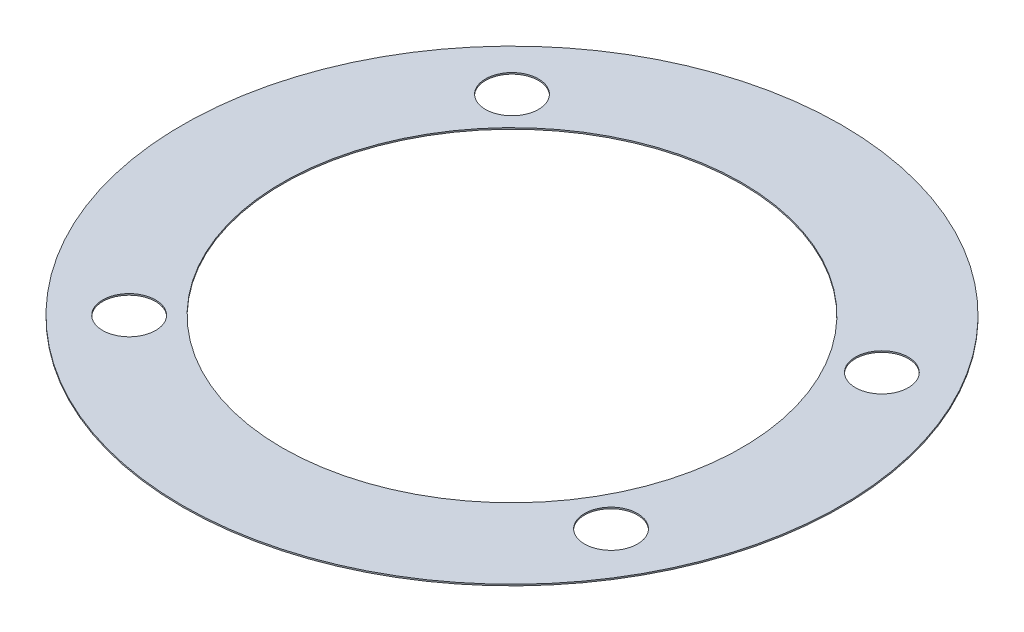
from build123d import *

# Parameters (mm, degrees)
SKETCH1_R                               = 88.9
SKETCH1_R_2                             = 61.975
BOSS_EXTRUDE1_DEPTH                     = 0.381
F_9_16_0_5625_DIAMETER_HOLE1_AT_2_COUNT = 2
F_9_16_0_5625_DIAMETER_HOLE1_AT_2_PITCH = 144.818259586


with BuildPart() as part:
    # Sketch1 → Boss-Extrude1 (new body)
    with BuildSketch(Plane(origin=(0, 0, 0), x_dir=(1, 0, 0), z_dir=(0, 1, 0))):
        with Locations(Location((0, 0, 0), (0, 0, 90))):
            Circle(SKETCH1_R)
        with Locations(Location((0, 0, 0), (0, 0, 90))):
            Circle(SKETCH1_R_2, mode=Mode.SUBTRACT)
    extrude(amount=BOSS_EXTRUDE1_DEPTH)

    # Sketch2 → 9/16 (0.5625) Diameter Hole1 (revolve, cut)
    with BuildSketch(Plane(origin=(-51.6382, 0.381, -51.64), x_dir=(0, 0, 1), z_dir=(1, 0, 0))):
        Polygon((0, 0), (0, 20.172398047), (7.14375, 15.88), (7.14375, 0), align=None)
    f_9_16_0_5625_diameter_hole1 = revolve(axis=Axis((-51.6382, 6.731, -51.64), (0, -1, 0)), mode=Mode.SUBTRACT)

    # 9/16 (0.5625) Diameter Hole1 at 2: 9/16 (0.5625) Diameter Hole1 ×2
    with Locations(*[Vector(0.7932991345710956, 0, 0.6088320647672483) * (i * F_9_16_0_5625_DIAMETER_HOLE1_AT_2_PITCH) for i in range(1, F_9_16_0_5625_DIAMETER_HOLE1_AT_2_COUNT)]):
        add(f_9_16_0_5625_diameter_hole1, mode=Mode.SUBTRACT)

    # Mirror1: 9/16 (0.5625) Diameter Hole1 across plane
    add(f_9_16_0_5625_diameter_hole1.mirror(Plane.XY), mode=Mode.SUBTRACT)

    # Mirror1 copy 1 sketch → Mirror1 copy 1 (revolve, cut)
    with BuildSketch(Plane(origin=(63.246, 0.381, -36.53), x_dir=(0, 0, -1), z_dir=(1, 0, 0))):
        Polygon((0, 0), (0, -20.172398047), (7.14375, -15.88), (7.14375, 0), align=None)
    revolve(axis=Axis((63.246, 6.731, -36.53), (0, 1, 0)), mode=Mode.SUBTRACT)


solid = part.part
